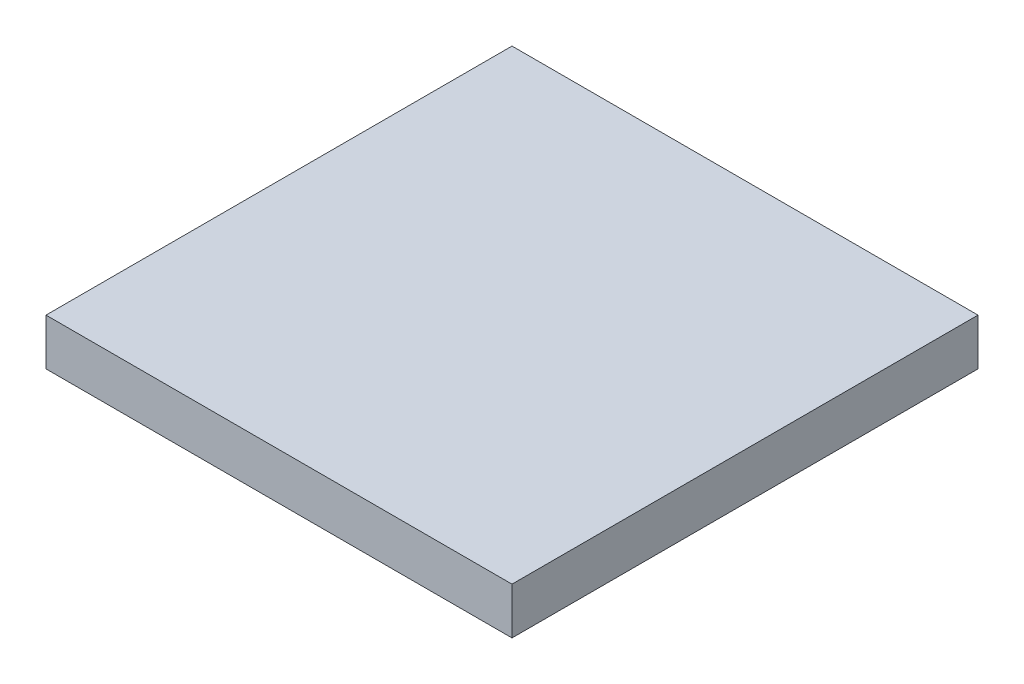
from build123d import *

# Parameters (mm, degrees)
SKETCH_1_W      = 500
SKETCH_1_H      = 500
EXTRUDE_1_DEPTH = 50


with BuildPart() as part:
    # 草图1 → 凸台-拉伸1 (new body)
    with BuildSketch(Plane(origin=(0, 0, 0), x_dir=(1, 0, 0), z_dir=(0, 1, 0))):
        Rectangle(SKETCH_1_W, SKETCH_1_H)
    extrude(amount=EXTRUDE_1_DEPTH)


solid = part.part
